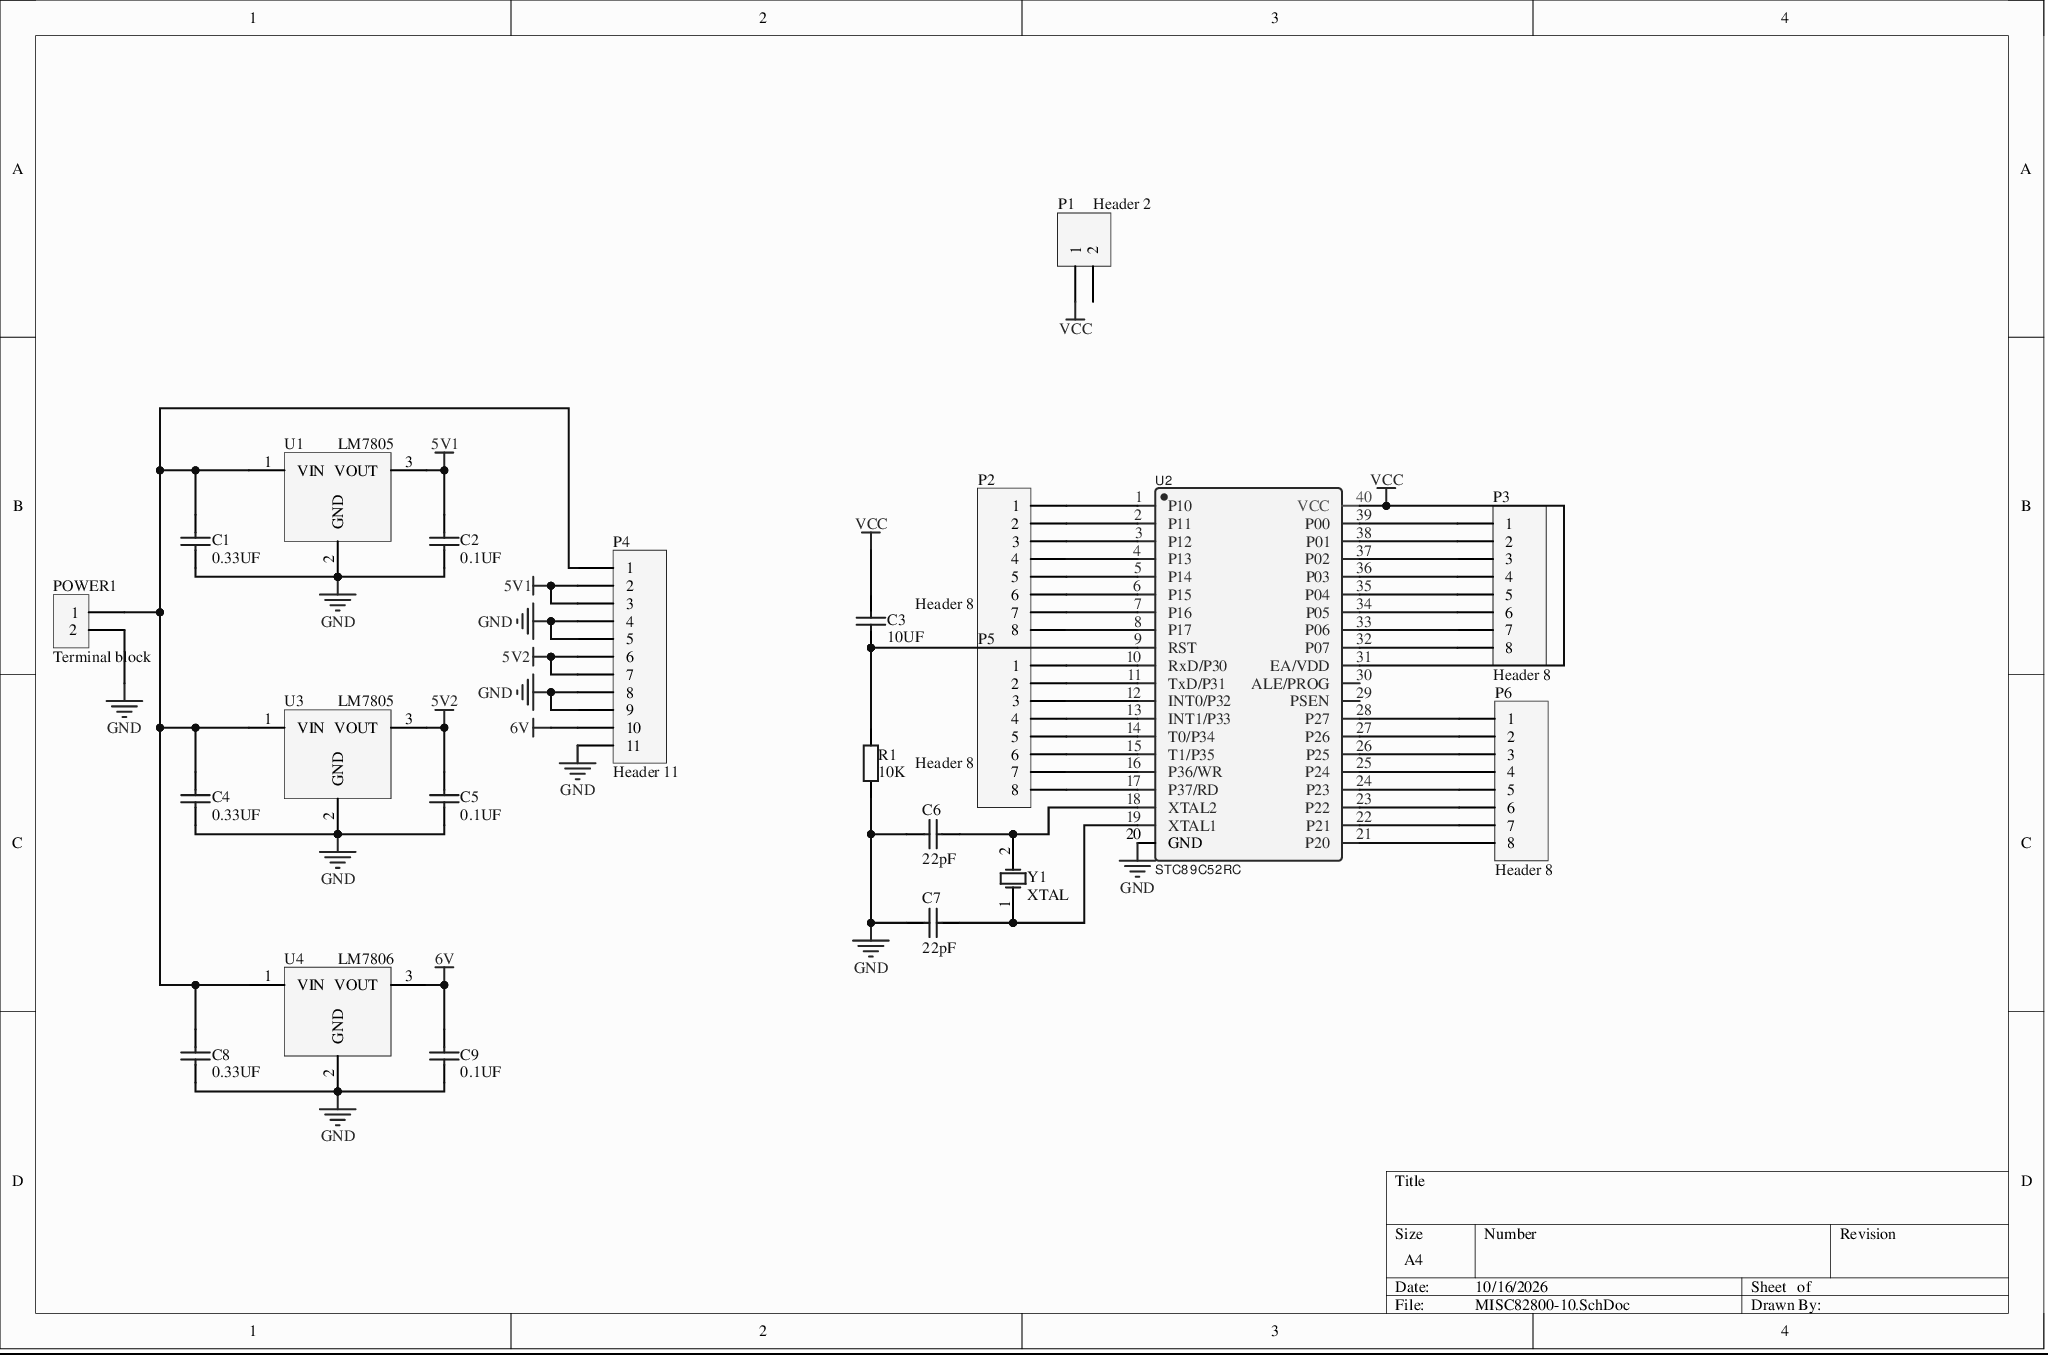
[diagram p0: MISC82800-10.SchDoc]
# Altium project MISC82800-3.PrjPcb
1 sheet, 22 parts. Net scope: global (net labels, ports and power ports of the same name join across sheets).
Board file: MISC82800.PcbDoc

## Sheet MISC82800-10.SchDoc
size A4

### Parts
C1  0.33UF  [RAD-0.3]
C2  0.1UF  [RAD-0.3]
C3  10UF  [RAD-0.3]
C4  0.33UF  [RAD-0.3]
C5  0.1UF  [RAD-0.3]
C6  22pF  [RAD-0.3]
C7  22pF  [RAD-0.3]
C8  0.33UF  [RAD-0.3]
C9  0.1UF  [RAD-0.3]
P1  Header 2  [HDR1X2]
P2  Header 8  [HDR1X8]
P3  Header 8  [HDR1X8]
P4  Header 11  [HDR1X11]
P5  Header 8  [HDR1X8]
P6  Header 8  [HDR1X8]
POWER1  Terminal block  [VH3.96-2A]
R1  10K  [AXIAL-0.4]
U1  LM7805  [TO220A]
U2  STC89C52RC  [STC89C52RC]
U3  LM7805  [TO220A]
U4  LM7806  [TO220A]
Y1  XTAL  [R38]

### Nets
5V1: C2.1 P4.2 P4.3 U1.3(VOUT)
5V2: C5.1 P4.6 P4.7 U3.3(VOUT)
6V: C9.1 P4.10 U4.3(VOUT)
GND: C1.2 C2.2 C4.2 C5.2 C6.2 C7.2 C8.2 C9.2 P4.4 P4.5 P4.8 P4.9 P4.11 POWER1.2 R1.1 U1.2(GND) U2.20(GND) U3.2(GND) U4.2(GND)
VCC: C3.1 P1.1 U2.31(EA/VDD) U2.40(VCC)
NetC1_1: C1.1 C4.1 C8.1 P4.1 POWER1.1 U1.1(VIN) U3.1(VIN) U4.1(VIN)
NetC3_2: C3.2 R1.2 U2.9(RST)
NetC6_1: C6.1 U2.18(XTAL2) Y1.2(OSC2)
NetC7_1: C7.1 U2.19(XTAL1) Y1.1(OSC1)
NetP2_1: P2.1 U2.1(P10)
NetP2_2: P2.2 U2.2(P11)
NetP2_3: P2.3 U2.3(P12)
NetP2_4: P2.4 U2.4(P13)
NetP2_5: P2.5 U2.5(P14)
NetP2_6: P2.6 U2.6(P15)
NetP2_7: P2.7 U2.7(P16)
NetP2_8: P2.8 U2.8(P17)
NetP3_1: P3.1 U2.39(P00)
NetP3_2: P3.2 U2.38(P01)
NetP3_3: P3.3 U2.37(P02)
NetP3_4: P3.4 U2.36(P03)
NetP3_5: P3.5 U2.35(P04)
NetP3_6: P3.6 U2.34(P05)
NetP3_7: P3.7 U2.33(P06)
NetP3_8: P3.8 U2.32(P07)
NetP5_1: P5.1 U2.10(RxD/P30)
NetP5_2: P5.2 U2.11(TxD/P31)
NetP5_3: P5.3 U2.12(INT0/P32)
NetP5_4: P5.4 U2.13(INT1/P33)
NetP5_5: P5.5 U2.14(T0/P34)
NetP5_6: P5.6 U2.15(T1/P35)
NetP5_7: P5.7 U2.16(P36/WR)
NetP5_8: P5.8 U2.17(P37/RD)
NetP6_1: P6.1 U2.28(P27)
NetP6_2: P6.2 U2.27(P26)
NetP6_3: P6.3 U2.26(P25)
NetP6_4: P6.4 U2.25(P24)
NetP6_5: P6.5 U2.24(P23)
NetP6_6: P6.6 U2.23(P22)
NetP6_7: P6.7 U2.22(P21)
NetP6_8: P6.8 U2.21(P20)

Not connected (* = marked no-connect by the designer): P1 2; U2 29(PSEN) 30(ALE/PROG)

### Library data of the parts
C1-C9 = Cap: Capacitor; Value: 100pF; Published: 8-Jun-2000; LatestRevisionDate: 17-Jul-2002; LatestRevisionNote: Re-released for DXP Platform.; PackageReference: RAD-0.3; PackageDescription: Radial Cap, Thru-Hole; 2 Leads; 0.3 in Pin Spacing; Publisher: COMPANY_A
P1 = Header 2: Header, 2-Pin; LatestRevisionDate: 17-Jul-2002; LatestRevisionNote: Re-released for DXP Platform.; Publisher: COMPANY_A
P2 P3 P5 P6 = Header 8: Header, 8-Pin; LatestRevisionDate: 17-Jul-2002; LatestRevisionNote: Re-released for DXP Platform.; Publisher: COMPANY_A
P4 = Header 11: Header, 11-Pin; LatestRevisionDate: 17-Jul-2002; LatestRevisionNote: Re-released for DXP Platform.; Publisher: COMPANY_A
POWER1 = VH2
R1 = Res2: Resistor; Value: 1K; Published: 8-Jun-2000; LatestRevisionDate: 17-Jul-2002; LatestRevisionNote: Re-released for DXP Platform.; PackageReference: AXIAL-0.4; PackageDescription: Axial Device, Thru-Hole; 2 Leads; 0.4 in Pin Spacing; Publisher: COMPANY_A
U4 = LM7805
Y1 = XTAL: Crystal Oscillator; Published: 8-Jun-2000; LatestRevisionDate: 17-Jul-2002; LatestRevisionNote: Re-released for DXP Platform.; PackageReference: R38; PackageDescription: Crystal, Thru-Hole; 2 Leads; Body 3.1 x 8.2 mm (Dia.xH); Publisher: COMPANY_A